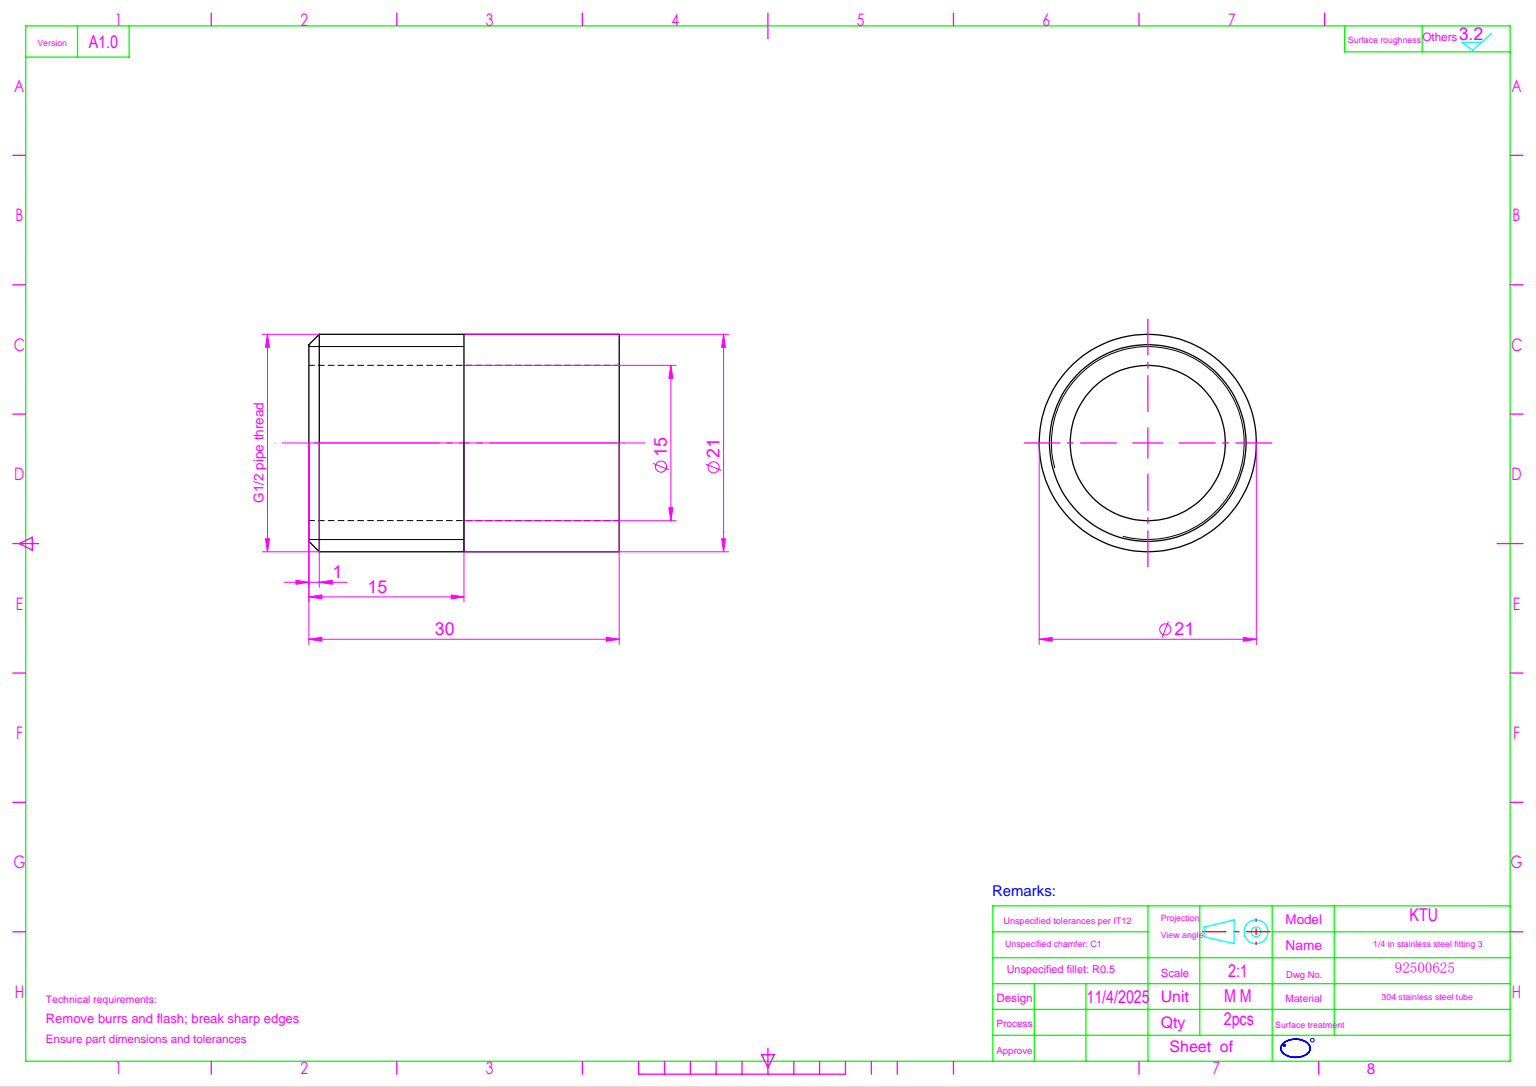
from build123d import *

# Parameters (mm, degrees)
SKETCH_1_R      = 10.5
SKETCH_1_R_2    = 7.5
EXTRUDE_1_DEPTH = 15
CHAMFER_1_SIZE  = 1


with BuildPart() as part:
    # 草图1 → 凸台-拉伸1 (new, symmetric)
    with BuildSketch(Plane(origin=(0, 0, 0), x_dir=(0, 0, -1), z_dir=(1, 0, 0))):
        Circle(SKETCH_1_R)
        Circle(SKETCH_1_R_2, mode=Mode.SUBTRACT)
    extrude(amount=EXTRUDE_1_DEPTH, both=True)

    # 倒角1
    chamfer_1_edges = [part.edges().sort_by_distance(p)[0] for p in [
        (15, 0, 10.5),
    ]]
    chamfer(chamfer_1_edges, length=CHAMFER_1_SIZE)


solid = part.part
